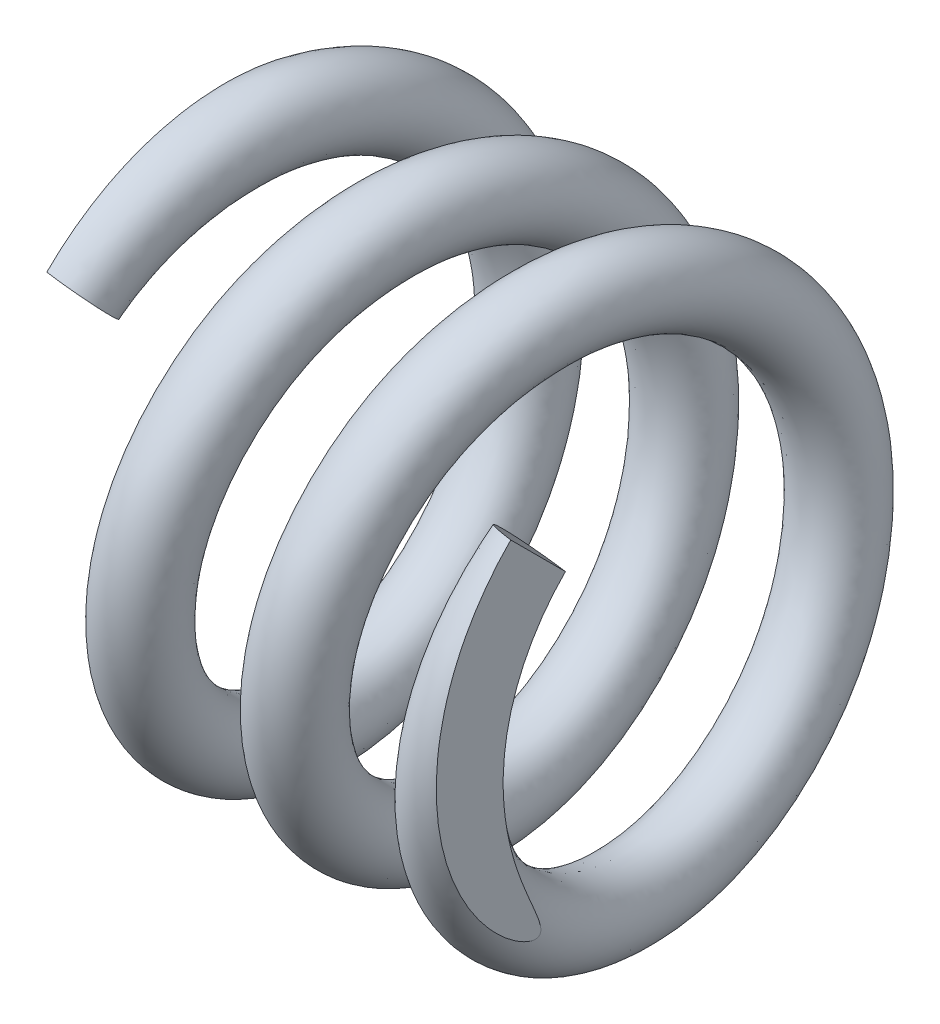
SolidWorks part; units mm, degrees
ref_plane "Front Plane" through (0, 0, 0) normal (0, 0, 1) x (1, 0, 0)
ref_plane "Top Plane" through (0, 0, 0) normal (0, 1, 0) x (1, 0, 0)
ref_plane "Right Plane" through (0, 0, 0) normal (1, 0, 0) x (0, 0, -1)
other "Configuration Table"
sketch "Sketch1" plane through (0, 0, 0) normal (1, 0, 0) x (0, 0, -1)
  circle A0 centre (0, 0) radius 1.5
  dimension "D1" = 3
curve "Helix/Spiral1" pitch 1 height 3 turns 3
sweep "Sweep1" add path "Helix/Spiral1" circular profile diameter 0.5 parameters "D3"=0.5
sketch "Sketch8" plane through (0, 0, 0) normal (0, 0, 1) x (1, 0, 0)
  line L1 (0, -2.7275) -> (3, -2.7275)
  line L2 (0, -2.7275) -> (0, 2.2803)
  line L3 (0, 2.2803) -> (3, 2.2803)
  line L4 (3, -2.7275) -> (3, 2.2803)
  line L5 (0, -2.7275) -> (3, 2.2803) construction
  line L6 (0, 2.2803) -> (3, -2.7275) construction
  point P0 (1.5, -0.2236)
  dimension "D1" = 3
extrude "Cut-Extrude2" cut sketch "Sketch8" against normal through all both and the other way through all flip side to cut
sketch "Sketch9" plane through (0, 0, 0) normal (1, 0, 0) x (0, 0, -1)
  circle A0 centre (0, 0) radius 1.265
